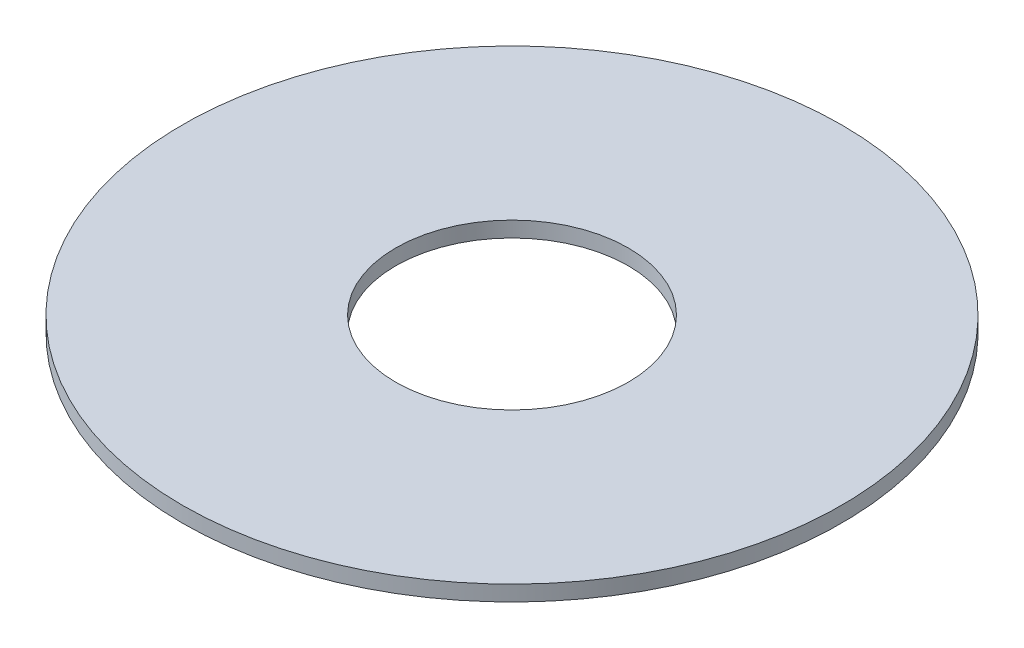
from build123d import *

# Parameters (mm, degrees)
SKETCH1_R           = 42.5
SKETCH1_R_2         = 15
BOSS_EXTRUDE1_DEPTH = 2


with BuildPart() as part:
    # Sketch1 → Boss-Extrude1 (new body)
    with BuildSketch(Plane(origin=(0, 0, 0), x_dir=(1, 0, 0), z_dir=(0, 1, 0))):
        with Locations(Location((0, 0, 0), (0, 0, 270))):
            Circle(SKETCH1_R)
        with Locations(Location((0, 0, 0), (0, 0, 270))):
            Circle(SKETCH1_R_2, mode=Mode.SUBTRACT)
    extrude(amount=BOSS_EXTRUDE1_DEPTH)


solid = part.part
